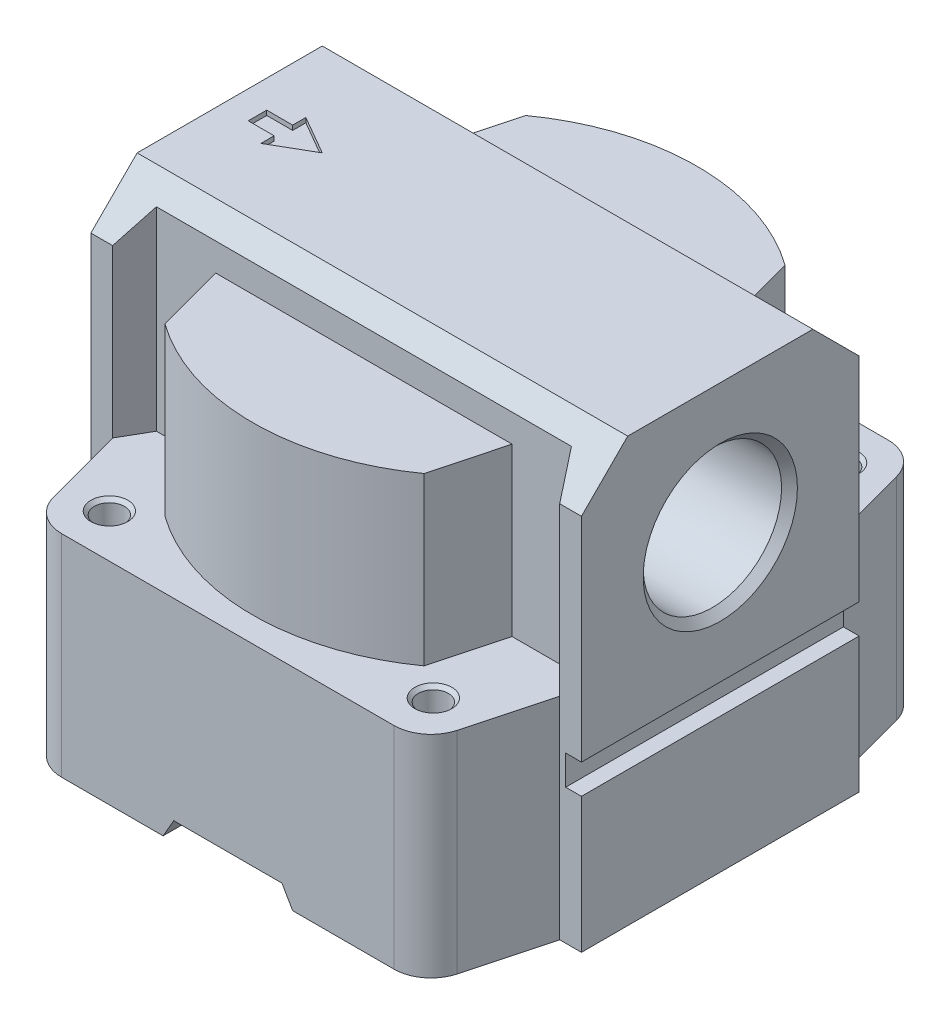
from build123d import *

# Parameters (mm, degrees)
EXTRUDE_1_DEPTH             = 22.8
EXTRUDE_2_DEPTH             = 45.8
CUT_EXTRUDE_1_DEPTH         = 26.5
CUT_EXTRUDE_1_DEPTH_BACK    = 26.5
EXTRUDE_3_DEPTH             = 40.8
CUT_EXTRUDE_2_DEPTH         = 26.7
CUT_EXTRUDE_2_DEPTH_BACK    = 26.7
SKETCH_5_W                  = 1.7
SKETCH_5_H                  = 3.2
CUT_EXTRUDE_3_DEPTH         = 26.7
CUT_EXTRUDE_3_DEPTH_BACK    = 26.7
SKETCH_6_W                  = 1.7
SKETCH_6_H                  = 3.2
HOLE_WIZARD_1_D             = 14.95
HOLE_WIZARD_1_DEPTH         = 11.7
HOLE_WIZARD_1_CSINK_D       = 16.662
HOLE_WIZARD_1_CSINK_ANGLE   = 90
HOLE_WIZARD_1_TIP           = 4.315693262
HOLE_WIZARD_2_D             = 14.95
HOLE_WIZARD_2_DEPTH         = 11.7
HOLE_WIZARD_2_CSINK_D       = 16.662
HOLE_WIZARD_2_CSINK_ANGLE   = 90
HOLE_WIZARD_2_TIP           = 4.315693262
PATTERN_LINEAR_1_COUNT      = 2
PATTERN_LINEAR_1_PITCH      = 44
PATTERN_LINEAR_1_COUNT_DIR2 = 2
PATTERN_LINEAR_1_PITCH_DIR2 = 35
CUT_EXTRUDE_4_DEPTH         = 0.5
CUT_EXTRUDE_5_DEPTH         = 26.7
CUT_EXTRUDE_5_DEPTH_BACK    = 26.7
SKETCH_16_W                 = 23
SKETCH_16_H                 = 2


with BuildPart() as part:
    # 草图1 → 凸台-拉伸1 (new body)
    with BuildSketch(Plane(origin=(0, -31.8, 0), x_dir=(1, 0, 0), z_dir=(0, 1, 0))):
        with BuildLine():
            Line((-24.15, -15), (-21.809389802, -23.73527618))
            ThreePointArc((-21.809389802, -23.73527618), (-20.380732213, -25.873413361), (-17.945686497, -26.7))
            Line((-17.945686497, -26.7), (17.945686497, -26.7))
            ThreePointArc((17.945686497, -26.7), (20.380732213, -25.873413361), (21.809389802, -23.73527618))
            Line((21.809389802, -23.73527618), (24.15, -15))
            Line((24.15, -15), (24.15, 15))
            Line((24.15, 15), (21.809389802, 23.73527618))
            ThreePointArc((21.809389802, 23.73527618), (20.380732213, 25.873413361), (17.945686497, 26.7))
            Line((17.945686497, 26.7), (-17.945686497, 26.7))
            ThreePointArc((-17.945686497, 26.7), (-20.380732213, 25.873413361), (-21.809389802, 23.73527618))
            Line((-21.809389802, 23.73527618), (-24.15, 15))
            Line((-24.15, 15), (-24.15, -15))
        make_face()
    extrude(amount=EXTRUDE_1_DEPTH)

    # 草图2 → 凸台-拉伸2 (add)
    with BuildSketch(Plane(origin=(0, -31.8, 0), x_dir=(1, 0, 0), z_dir=(0, 1, 0))):
        Polygon((-26.5, -15), (-24.15, -15), (-22.417949192, -12), (22.417949192, -12), (24.15, -15), (26.5, -15), (26.5, 15), (24.15, 15), (22.417949192, 12), (-22.417949192, 12), (-24.15, 15), (-26.5, 15), align=None)
    extrude(amount=EXTRUDE_2_DEPTH)

    # 草图3 → 切除-拉伸1 (cut, two sides: drawn at the far end of the back side and taken through both)
    with BuildSketch(Plane(origin=(0, 0, 0), x_dir=(0, 0, -1), z_dir=(1, 0, 0)).offset(-CUT_EXTRUDE_1_DEPTH_BACK)):
        Polygon((-26.7, 19), (-26.7, 0), (-15, 0), (-15, 9), (-10, 14), (10, 14), (15, 9), (15, 0), (26.7, 0), (26.7, 19), align=None)
    extrude(amount=CUT_EXTRUDE_1_DEPTH + CUT_EXTRUDE_1_DEPTH_BACK, mode=Mode.SUBTRACT)

    # 草图4 → 凸台-拉伸3 (add)
    with BuildSketch(Plane(origin=(0, -31.8, 0), x_dir=(1, 0, 0), z_dir=(0, 1, 0))):
        with BuildLine():
            Line((-16, -12), (-14.002114735, -19.492069745))
            ThreePointArc((-14.002114735, -19.492069745), (0, -24), (14.002114735, -19.492069745))
            Line((14.002114735, -19.492069745), (16, -12))
            Line((16, -12), (16, 12))
            Line((16, 12), (14.002114735, 19.492069745))
            ThreePointArc((14.002114735, 19.492069745), (0, 24), (-14.002114735, 19.492069745))
            Line((-14.002114735, 19.492069745), (-16, 12))
            Line((-16, 12), (-16, -12))
        make_face()
    extrude(amount=EXTRUDE_3_DEPTH)

    # 草图5 → 切除-拉伸2 (cut, two sides: drawn at the far end of the back side and taken through both)
    with BuildSketch(Plane.XY.offset(-CUT_EXTRUDE_2_DEPTH_BACK)):
        with Locations((25.65, -15.6)):
            Rectangle(SKETCH_5_W, SKETCH_5_H)
    extrude(amount=CUT_EXTRUDE_2_DEPTH + CUT_EXTRUDE_2_DEPTH_BACK, mode=Mode.SUBTRACT)

    # 草图6 → 切除-拉伸3 (cut, two sides: drawn at the far end of the back side and taken through both)
    with BuildSketch(Plane.XY.offset(-CUT_EXTRUDE_3_DEPTH_BACK)):
        with Locations((-25.65, -15.6)):
            Rectangle(SKETCH_6_W, SKETCH_6_H)
    extrude(amount=CUT_EXTRUDE_3_DEPTH + CUT_EXTRUDE_3_DEPTH_BACK, mode=Mode.SUBTRACT)

    # 孔1
    with Locations(Plane(origin=(26.5, 0, 0), x_dir=(0, 0, -1), z_dir=(1, 0, 0))):
        with Locations((0, 0)):
            CounterSinkHole(HOLE_WIZARD_1_D / 2, HOLE_WIZARD_1_CSINK_D / 2, depth=HOLE_WIZARD_1_DEPTH, counter_sink_angle=HOLE_WIZARD_1_CSINK_ANGLE)
            with Locations((0, 0, -(HOLE_WIZARD_1_DEPTH + HOLE_WIZARD_1_TIP / 2))):  # 120° drill point
                Cone(0, HOLE_WIZARD_1_D / 2, HOLE_WIZARD_1_TIP, mode=Mode.SUBTRACT)

    # 孔2
    with Locations(Plane.ZY.offset(26.5)):
        with Locations((0, 0)):
            CounterSinkHole(HOLE_WIZARD_2_D / 2, HOLE_WIZARD_2_CSINK_D / 2, depth=HOLE_WIZARD_2_DEPTH, counter_sink_angle=HOLE_WIZARD_2_CSINK_ANGLE)
            with Locations((0, 0, -(HOLE_WIZARD_2_DEPTH + HOLE_WIZARD_2_TIP / 2))):  # 120° drill point
                Cone(0, HOLE_WIZARD_2_D / 2, HOLE_WIZARD_2_TIP, mode=Mode.SUBTRACT)

    # 草图11 → 孔3 (revolve, cut)
    with BuildSketch(Plane(origin=(17.5, -9, 22), x_dir=(0, 0, 1), z_dir=(1, 0, 0))):
        Polygon((0, 0), (0, 4.935884786), (1.621, 4), (1.621, 0.379), (2, 0), align=None)
    hole_wizard_3 = revolve(axis=Axis((17.5, 5.308894879, 22), (0, -1, 0)), mode=Mode.SUBTRACT)

    # 阵列(线性)1: Hole Wizard 3 2 × 2
    with Locations(*[(-j * PATTERN_LINEAR_1_PITCH_DIR2, 0, -i * PATTERN_LINEAR_1_PITCH) for i in range(PATTERN_LINEAR_1_COUNT) for j in range(PATTERN_LINEAR_1_COUNT_DIR2) if (i, j) != (0, 0)]):
        add(hole_wizard_3, mode=Mode.SUBTRACT)

    # 草图14 → 切除-拉伸4 (cut)
    with BuildSketch(Plane(origin=(0, 14, 0), x_dir=(1, 0, 0), z_dir=(0, 1, 0))):
        Polygon((-23.5, -1), (-20.7, -1), (-20.7, -2.424871131), (-16.5, 0), (-20.7, 2.424871131), (-20.7, 1), (-23.5, 1), align=None)
    extrude(amount=-CUT_EXTRUDE_4_DEPTH, mode=Mode.SUBTRACT)

    # 草图15 → 切除-拉伸5 (cut, two sides: drawn at the far end of the back side and taken through both)
    with BuildSketch(Plane.XY.offset(-CUT_EXTRUDE_5_DEPTH_BACK)):
        Polygon((-7, -31.8), (7, -31.8), (5.845299462, -29.8), (-5.845299462, -29.8), align=None)
    extrude(amount=CUT_EXTRUDE_5_DEPTH + CUT_EXTRUDE_5_DEPTH_BACK, mode=Mode.SUBTRACT)

    # 草图16 → 旋转1 (revolve)
    with BuildSketch(Plane.XY):
        with Locations((11.5, -30.8)):
            Rectangle(SKETCH_16_W, SKETCH_16_H)
    revolve(axis=Axis((0, -31.8, 0), (0, 1, 0)))


solid = part.part
